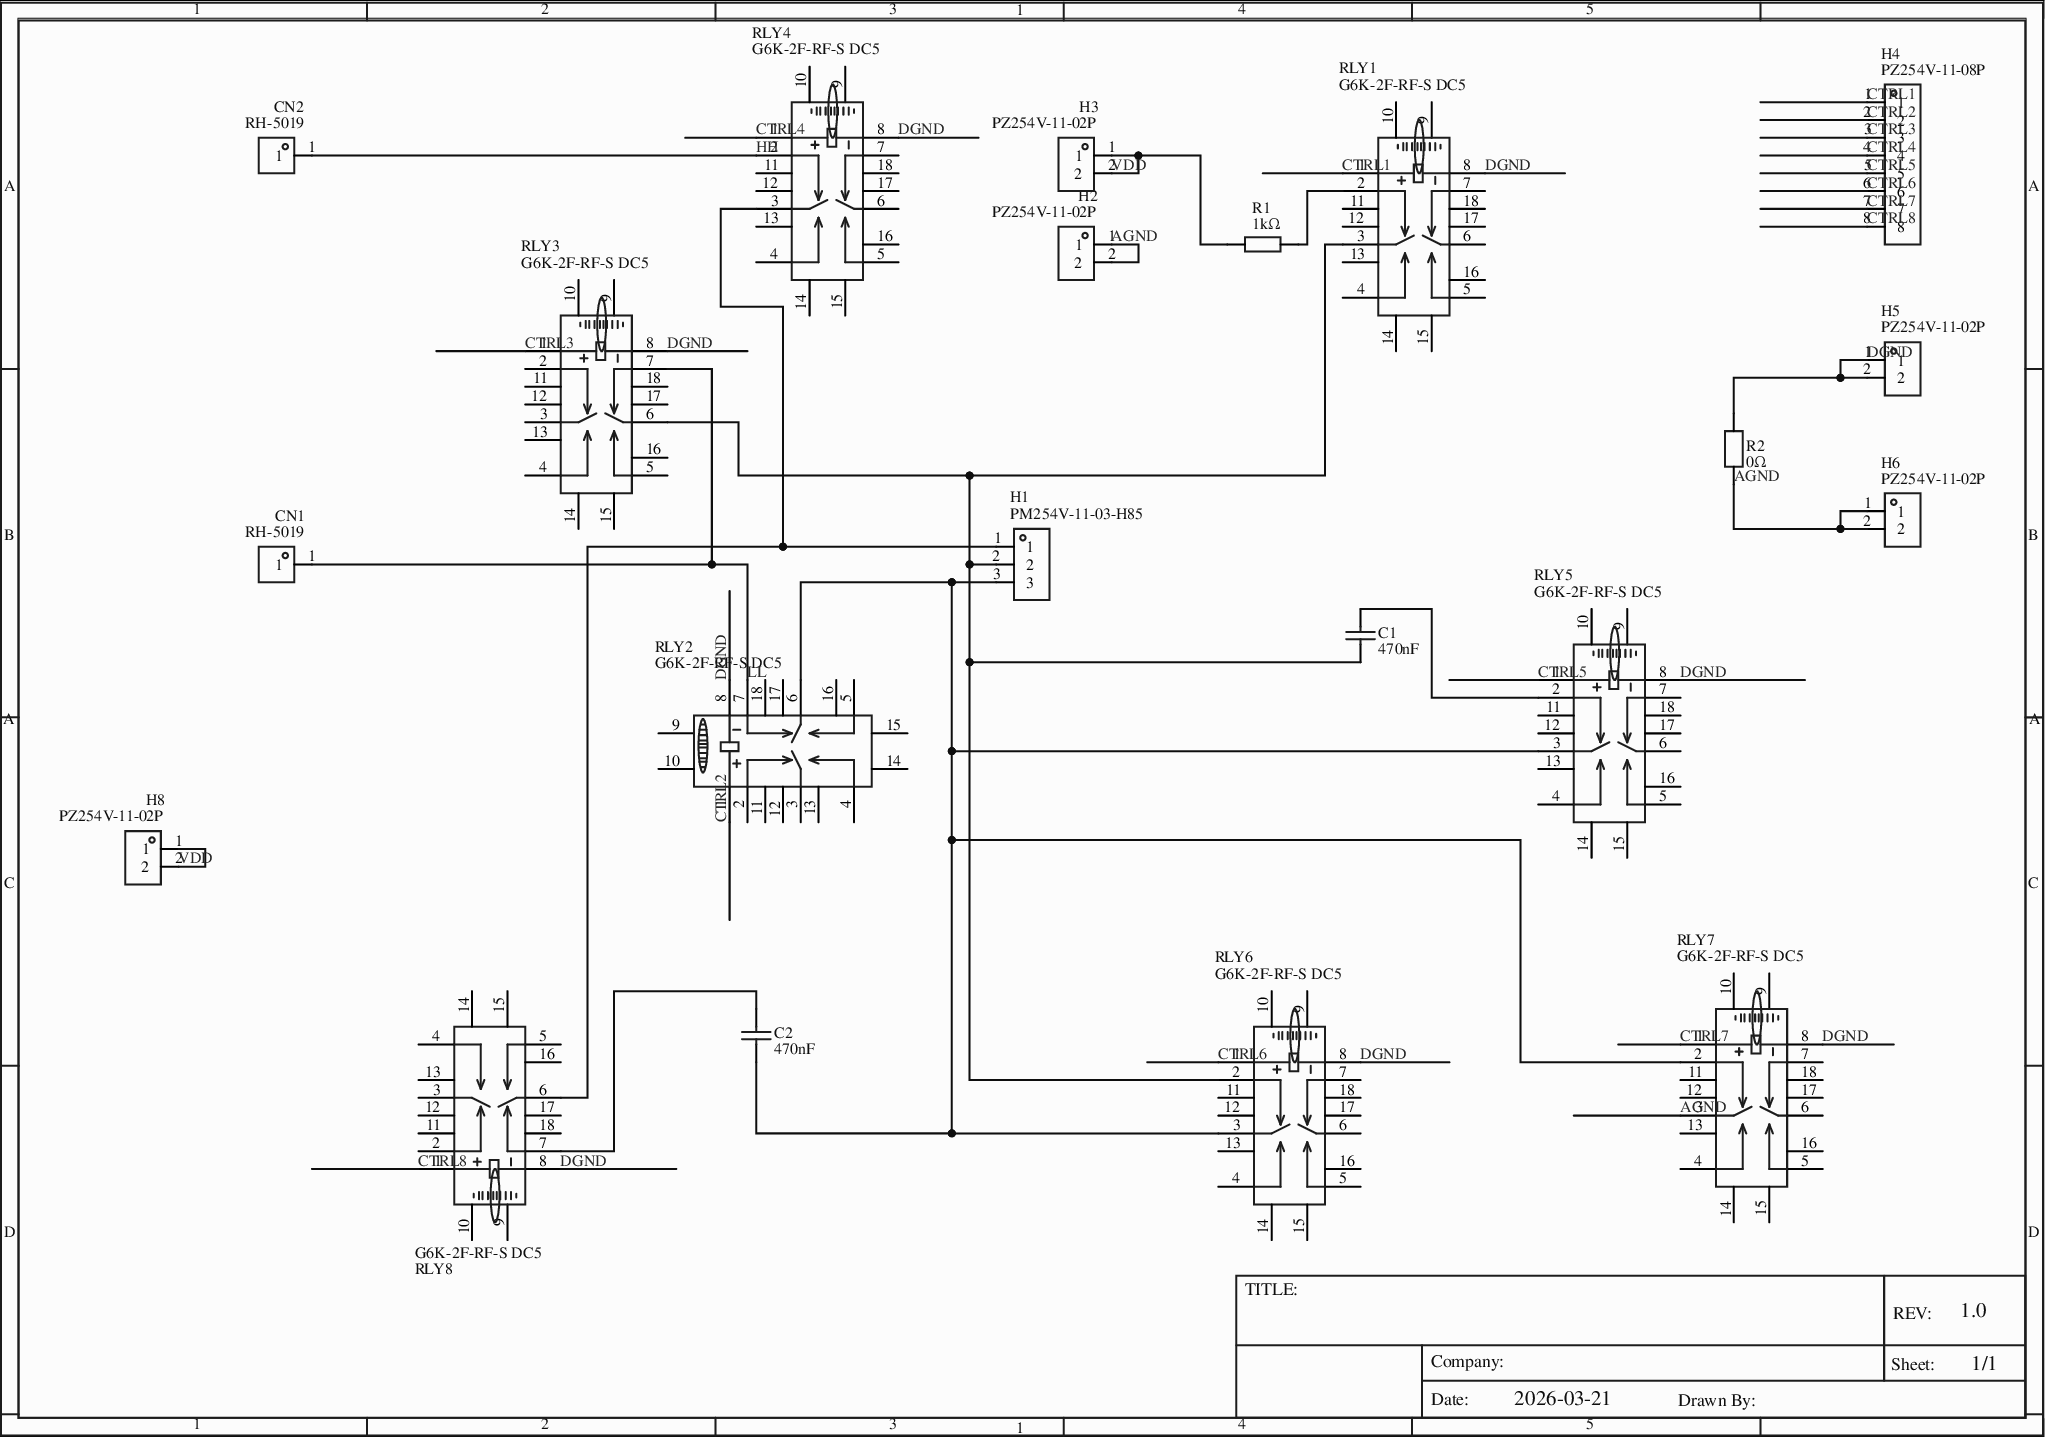
[diagram p0: MISC51843-3.schdoc]
# Altium project MISC51843-2.PrjPcb
1 sheet, 21 parts. Net scope: global (net labels, ports and power ports of the same name join across sheets).
Board file: MISC51843.pcbdoc

## Sheet MISC51843-3.schdoc
size 292 x 205 mm; Name: MISC51843; @Project Name: MISC51843; REV: 1.0; Date: 2026-03-21; Sheet: 1/1; Manufacturer Part: ?

### Parts
C1  470nF  [C0805]
C2  470nF  [C0805]
CN1  RH-5019  [TESTPOINT-SMD_L3.8-W2.0_RH-5019]
CN2  RH-5019  [TESTPOINT-SMD_L3.8-W2.0_RH-5019]
H1  PM254V-11-03-H85  [HDR-TH_3P-P2.54-V-F]
H2  PZ254V-11-02P  [HDR-TH_2P-P2.54-V-M]
H3  PZ254V-11-02P  [HDR-TH_2P-P2.54-V-M]
H4  PZ254V-11-08P  [HDR-TH_8P-P2.54-V-M]
H5  PZ254V-11-02P  [HDR-TH_2P-P2.54-V-M]
H6  PZ254V-11-02P  [HDR-TH_2P-P2.54-V-M]
H8  PZ254V-11-02P  [HDR-TH_2P-P2.54-V-M]
R1  1kΩ  [R1210]
R2  0Ω  [R1206]
RLY1  G6K-2F-RF-S DC5  [RELAY-SMD_G6K-2F-RF-S-DC12]
RLY2  G6K-2F-RF-S DC5  [RELAY-SMD_G6K-2F-RF-S-DC12]
RLY3  G6K-2F-RF-S DC5  [RELAY-SMD_G6K-2F-RF-S-DC12]
RLY4  G6K-2F-RF-S DC5  [RELAY-SMD_G6K-2F-RF-S-DC12]
RLY5  G6K-2F-RF-S DC5  [RELAY-SMD_G6K-2F-RF-S-DC12]
RLY6  G6K-2F-RF-S DC5  [RELAY-SMD_G6K-2F-RF-S-DC12]
RLY7  G6K-2F-RF-S DC5  [RELAY-SMD_G6K-2F-RF-S-DC12]
RLY8  G6K-2F-RF-S DC5  [RELAY-SMD_G6K-2F-RF-S-DC12]

### Nets
AGND: H2.1 H2.2 H6.1 H6.2 R2.1 RLY7.3
CTRL1: H4.1 RLY1.1
CTRL2: H4.2 RLY2.1
CTRL3: H4.3 RLY3.1
CTRL4: H4.4 RLY4.1
CTRL5: H4.5 RLY5.1
CTRL6: H4.6 RLY6.1
CTRL7: H4.7 RLY7.1
CTRL8: H4.8 RLY8.1
DGND: H5.1 H5.2 R2.2 RLY1.8 RLY2.8 RLY3.8 RLY4.8 RLY5.8 RLY6.8 RLY7.8 RLY8.8
HH: CN2.1 RLY4.2
LL: CN1.1 RLY2.7 RLY3.7
VDD: H3.1 H3.2 H8.1 H8.2 R1.1
NetC1_1: C1.1 H1.2 RLY1.3 RLY3.6 RLY6.2
NetC1_2: C1.2 RLY5.2
NetC2_1: C2.1 H1.3 RLY2.6 RLY5.3 RLY6.3 RLY7.2
NetC2_2: C2.2 RLY8.7
NetH1_1: H1.1 RLY4.3 RLY8.6
NetR1_2: R1.2 RLY1.2

Not connected (* = marked no-connect by the designer): RLY1 4 5 6 7 9(SHELL) 10(SHELL) 11(SHELL) 12(SHELL) 13(SHELL) 14(SHELL) 15(9) 16(10) 17(11) 18(12); RLY2 2 3 4 5 9(SHELL) 10(SHELL) 11(SHELL) 12(SHELL) 13(SHELL) 14(SHELL) 15(9) 16(10) 17(11) 18(12); RLY3 2 3 4 5 9(SHELL) 10(SHELL) 11(SHELL) 12(SHELL) 13(SHELL) 14(SHELL) 15(9) 16(10) 17(11) 18(12); RLY4 4 5 6 7 9(SHELL) 10(SHELL) 11(SHELL) 12(SHELL) 13(SHELL) 14(SHELL) 15(9) 16(10) 17(11) 18(12); RLY5 4 5 6 7 9(SHELL) 10(SHELL) 11(SHELL) 12(SHELL) 13(SHELL) 14(SHELL) 15(9) 16(10) 17(11) 18(12); RLY6 4 5 6 7 9(SHELL) 10(SHELL) 11(SHELL) 12(SHELL) 13(SHELL) 14(SHELL) 15(9) 16(10) 17(11) 18(12); RLY7 4 5 6 7 9(SHELL) 10(SHELL) 11(SHELL) 12(SHELL) 13(SHELL) 14(SHELL) 15(9) 16(10) 17(11) 18(12); RLY8 2 3 4 5 9(SHELL) 10(SHELL) 11(SHELL) 12(SHELL) 13(SHELL) 14(SHELL) 15(9) 16(10) 17(11) 18(12)

### Notes on the sheet
- 1
- 2
- 3
- 4
- 5
- A
- B
- C
- D
- TITLE:
- Company:
- Sheet:
- REV:
- 1.0
- 1/1
- Date:
- 2026-03-21
- Drawn By:

### Library data of the parts
C1 = CL21B474KBFNNNE: Manufacturer: SAMSUNG(三星); Convert to PCB: yes; UniqueId: gge4bc09f60449cdcb3; Device: CL21B474KBFNNNE; Supplier: LCSC; Manufacturer Part: CL21B474KBFNNNE; Supplier Part: C13967; JLCPCB Part Class: Basic Part; Add into BOM: yes; Origin Footprint: C0805; SymbolName: 470nF; FootprintName: C0805
C2 = CL21B474KBFNNNE: Manufacturer: SAMSUNG(三星); Convert to PCB: yes; UniqueId: ggeccc321c5639fa0de; Device: CL21B474KBFNNNE; Supplier: LCSC; Manufacturer Part: CL21B474KBFNNNE; Supplier Part: C13967; JLCPCB Part Class: Basic Part; Add into BOM: yes; Origin Footprint: C0805; SymbolName: 470nF; FootprintName: C0805
CN1 = RH-5019: Manufacturer: 荣和; Convert to PCB: yes; UniqueId: gge7fc6a1c0fa59964e; ModelId: c020184594ef49cc9f8a46377413b7a6; Device: RH-5019; Supplier: LCSC; Supplier Part: C5199800; Manufacturer Part: RH-5019; JLCPCB Part Class: Extended Part; Add into BOM: yes; Origin Footprint: TESTPOINT-SMD_L3.8-W2.0_RH-5019; SymbolName: RH-5019; FootprintName: TESTPOINT-SMD_L3.8-W2.0_RH-5019; ModelName: TESTPOINT-SMD_L3.8-W2.0_RH-5019
CN2 = RH-5019: Manufacturer: 荣和; Convert to PCB: yes; UniqueId: ggee236267680e07397; ModelId: c020184594ef49cc9f8a46377413b7a6; Device: RH-5019; Supplier: LCSC; Supplier Part: C5199800; Manufacturer Part: RH-5019; JLCPCB Part Class: Extended Part; Add into BOM: yes; Origin Footprint: TESTPOINT-SMD_L3.8-W2.0_RH-5019; SymbolName: RH-5019; FootprintName: TESTPOINT-SMD_L3.8-W2.0_RH-5019; ModelName: TESTPOINT-SMD_L3.8-W2.0_RH-5019
H1 = PM254V-11-03-H85: Manufacturer: XFCN(兴飞); Convert to PCB: yes; UniqueId: gge72f7cac46e8615be; Device: PM254V-11-03-H85; Supplier: LCSC; Supplier Part: C541850; Manufacturer Part: PM254V-11-03-H85; JLCPCB Part Class: Extended Part; Add into BOM: yes; Origin Footprint: HDR-TH_3P-P2.54-V-F; SymbolName: PM254V-11-03-H85; FootprintName: HDR-TH_3P-P2.54-V-F
H2 = PZ254V-11-02P: Manufacturer: XFCN(兴飞); Convert to PCB: yes; UniqueId: ggef9e9a0185bba7f95; Device: PZ254V-11-02P; Supplier: LCSC; Supplier Part: C492401; Manufacturer Part: PZ254V-11-02P; JLCPCB Part Class: Extended Part; Add into BOM: yes; Origin Footprint: HDR-TH_2P-P2.54-V-M; SymbolName: PZ254V-11-02P; FootprintName: HDR-TH_2P-P2.54-V-M
H3 = PZ254V-11-02P: Manufacturer: XFCN(兴飞); Convert to PCB: yes; UniqueId: gge6f8671641895d11a; Device: PZ254V-11-02P; Supplier: LCSC; Supplier Part: C492401; Manufacturer Part: PZ254V-11-02P; JLCPCB Part Class: Extended Part; Add into BOM: yes; Origin Footprint: HDR-TH_2P-P2.54-V-M; SymbolName: PZ254V-11-02P; FootprintName: HDR-TH_2P-P2.54-V-M
H4 = PZ254V-11-08P: Manufacturer: XFCN(兴飞); Convert to PCB: yes; UniqueId: gge64c0f90843b550c5; ModelId: f5b96e27511e49e38545e53df2320202; Device: PZ254V-11-08P; Supplier: LCSC; Supplier Part: C492407; Manufacturer Part: PZ254V-11-08P; JLCPCB Part Class: Extended Part; Add into BOM: yes; Origin Footprint: HDR-TH_8P-P2.54-V-M; SymbolName: PZ254V-11-08P; FootprintName: HDR-TH_8P-P2.54-V-M; ModelName: HDR-TH_8P-P2.54-V-M
H5 = PZ254V-11-02P: Manufacturer: XFCN(兴飞); Convert to PCB: yes; UniqueId: gge31f59832f20397a2; Device: PZ254V-11-02P; Supplier: LCSC; Supplier Part: C492401; Manufacturer Part: PZ254V-11-02P; JLCPCB Part Class: Extended Part; Add into BOM: yes; Origin Footprint: HDR-TH_2P-P2.54-V-M; SymbolName: PZ254V-11-02P; FootprintName: HDR-TH_2P-P2.54-V-M
H6 = PZ254V-11-02P: Manufacturer: XFCN(兴飞); Convert to PCB: yes; UniqueId: gge8e72c5a1d865cb32; Device: PZ254V-11-02P; Supplier: LCSC; Supplier Part: C492401; Manufacturer Part: PZ254V-11-02P; JLCPCB Part Class: Extended Part; Add into BOM: yes; Origin Footprint: HDR-TH_2P-P2.54-V-M; SymbolName: PZ254V-11-02P; FootprintName: HDR-TH_2P-P2.54-V-M
H8 = PZ254V-11-02P: Manufacturer: XFCN(兴飞); Convert to PCB: yes; UniqueId: gge81d141f822a2e72a; Device: PZ254V-11-02P; Supplier: LCSC; Supplier Part: C492401; Manufacturer Part: PZ254V-11-02P; JLCPCB Part Class: Extended Part; Add into BOM: yes; Origin Footprint: HDR-TH_2P-P2.54-V-M; SymbolName: PZ254V-11-02P; FootprintName: HDR-TH_2P-P2.54-V-M
R1 = 1210W2J0102T5E: Manufacturer: UNI-ROYAL(厚声); Convert to PCB: yes; UniqueId: ggebd22175f7292284d; Device: 1210W2J0102T5E; Supplier: LCSC; Supplier Part: C270888; Manufacturer Part: 1210W2J0102T5E; JLCPCB Part Class: Extended Part; Add into BOM: yes; Origin Footprint: R1210; SymbolName: 1kΩ; FootprintName: R1210
R2 = RE1206F1R000: Manufacturer: JIERR(捷而瑞); Convert to PCB: yes; UniqueId: ggeb2efdb6ff1147088; Device: RE1206F1R000; Supplier: LCSC; Supplier Part: C46961765; Manufacturer Part: RE1206F1R000; JLCPCB Part Class: Extended Part; Add into BOM: yes; Origin Footprint: R1206; SymbolName: 0Ω; FootprintName: R1206
RLY1 = G6K-2F-RF-S DC5: Manufacturer: OMRON(欧姆龙); Convert to PCB: yes; UniqueId: gge99e9a6d1fe0d2417; ModelId: 4ceb3aef9d064fc2ab47c1f22decd9f6; Device: G6K-2F-RF-S DC5; Supplier: LCSC; Supplier Part: C2750987; Manufacturer Part: G6K-2F-RF-S DC5; JLCPCB Part Class: Extended Part; Add into BOM: yes; Origin Footprint: RELAY-SMD_G6K-2F-RF-S-DC12; SymbolName: G6K-2F-RF-S DC5; FootprintName: RELAY-SMD_G6K-2F-RF-S-DC12; ModelName: RELAY-SMD_G6K-2F-RF-S-DC12
RLY2 = G6K-2F-RF-S DC5: Manufacturer: OMRON(欧姆龙); Convert to PCB: yes; UniqueId: gge34bc72b43afd4cd1; ModelId: 4ceb3aef9d064fc2ab47c1f22decd9f6; Device: G6K-2F-RF-S DC5; Supplier: LCSC; Supplier Part: C2750987; Manufacturer Part: G6K-2F-RF-S DC5; JLCPCB Part Class: Extended Part; Add into BOM: yes; Origin Footprint: RELAY-SMD_G6K-2F-RF-S-DC12; SymbolName: G6K-2F-RF-S DC5; FootprintName: RELAY-SMD_G6K-2F-RF-S-DC12; ModelName: RELAY-SMD_G6K-2F-RF-S-DC12
RLY3 = G6K-2F-RF-S DC5: Manufacturer: OMRON(欧姆龙); Convert to PCB: yes; UniqueId: gge88e37c47efcf9865; ModelId: 4ceb3aef9d064fc2ab47c1f22decd9f6; Device: G6K-2F-RF-S DC5; Supplier: LCSC; Supplier Part: C2750987; Manufacturer Part: G6K-2F-RF-S DC5; JLCPCB Part Class: Extended Part; Add into BOM: yes; Origin Footprint: RELAY-SMD_G6K-2F-RF-S-DC12; SymbolName: G6K-2F-RF-S DC5; FootprintName: RELAY-SMD_G6K-2F-RF-S-DC12; ModelName: RELAY-SMD_G6K-2F-RF-S-DC12
RLY4 = G6K-2F-RF-S DC5: Manufacturer: OMRON(欧姆龙); Convert to PCB: yes; UniqueId: ggef4119901c794c351; ModelId: 4ceb3aef9d064fc2ab47c1f22decd9f6; Device: G6K-2F-RF-S DC5; Supplier: LCSC; Supplier Part: C2750987; Manufacturer Part: G6K-2F-RF-S DC5; JLCPCB Part Class: Extended Part; Add into BOM: yes; Origin Footprint: RELAY-SMD_G6K-2F-RF-S-DC12; SymbolName: G6K-2F-RF-S DC5; FootprintName: RELAY-SMD_G6K-2F-RF-S-DC12; ModelName: RELAY-SMD_G6K-2F-RF-S-DC12
RLY5 = G6K-2F-RF-S DC5: Manufacturer: OMRON(欧姆龙); Convert to PCB: yes; UniqueId: gge0e51ede8c4fc8b0f; ModelId: 4ceb3aef9d064fc2ab47c1f22decd9f6; Device: G6K-2F-RF-S DC5; Supplier: LCSC; Supplier Part: C2750987; Manufacturer Part: G6K-2F-RF-S DC5; JLCPCB Part Class: Extended Part; Add into BOM: yes; Origin Footprint: RELAY-SMD_G6K-2F-RF-S-DC12; SymbolName: G6K-2F-RF-S DC5; FootprintName: RELAY-SMD_G6K-2F-RF-S-DC12; ModelName: RELAY-SMD_G6K-2F-RF-S-DC12
RLY6 = G6K-2F-RF-S DC5: Manufacturer: OMRON(欧姆龙); Convert to PCB: yes; UniqueId: gge039e2dbc65126126; ModelId: 4ceb3aef9d064fc2ab47c1f22decd9f6; Device: G6K-2F-RF-S DC5; Supplier: LCSC; Supplier Part: C2750987; Manufacturer Part: G6K-2F-RF-S DC5; JLCPCB Part Class: Extended Part; Add into BOM: yes; Origin Footprint: RELAY-SMD_G6K-2F-RF-S-DC12; SymbolName: G6K-2F-RF-S DC5; FootprintName: RELAY-SMD_G6K-2F-RF-S-DC12; ModelName: RELAY-SMD_G6K-2F-RF-S-DC12
RLY7 = G6K-2F-RF-S DC5: Manufacturer: OMRON(欧姆龙); Convert to PCB: yes; UniqueId: gge2967527e3f935921; ModelId: 4ceb3aef9d064fc2ab47c1f22decd9f6; Device: G6K-2F-RF-S DC5; Supplier: LCSC; Supplier Part: C2750987; Manufacturer Part: G6K-2F-RF-S DC5; JLCPCB Part Class: Extended Part; Add into BOM: yes; Origin Footprint: RELAY-SMD_G6K-2F-RF-S-DC12; SymbolName: G6K-2F-RF-S DC5; FootprintName: RELAY-SMD_G6K-2F-RF-S-DC12; ModelName: RELAY-SMD_G6K-2F-RF-S-DC12
RLY8 = G6K-2F-RF-S DC5: Manufacturer: OMRON(欧姆龙); Convert to PCB: yes; UniqueId: gge584f8b22a76c1d9c; ModelId: 4ceb3aef9d064fc2ab47c1f22decd9f6; Device: G6K-2F-RF-S DC5; Supplier: LCSC; Supplier Part: C2750987; Manufacturer Part: G6K-2F-RF-S DC5; JLCPCB Part Class: Extended Part; Add into BOM: yes; Origin Footprint: RELAY-SMD_G6K-2F-RF-S-DC12; SymbolName: G6K-2F-RF-S DC5; FootprintName: RELAY-SMD_G6K-2F-RF-S-DC12; ModelName: RELAY-SMD_G6K-2F-RF-S-DC12